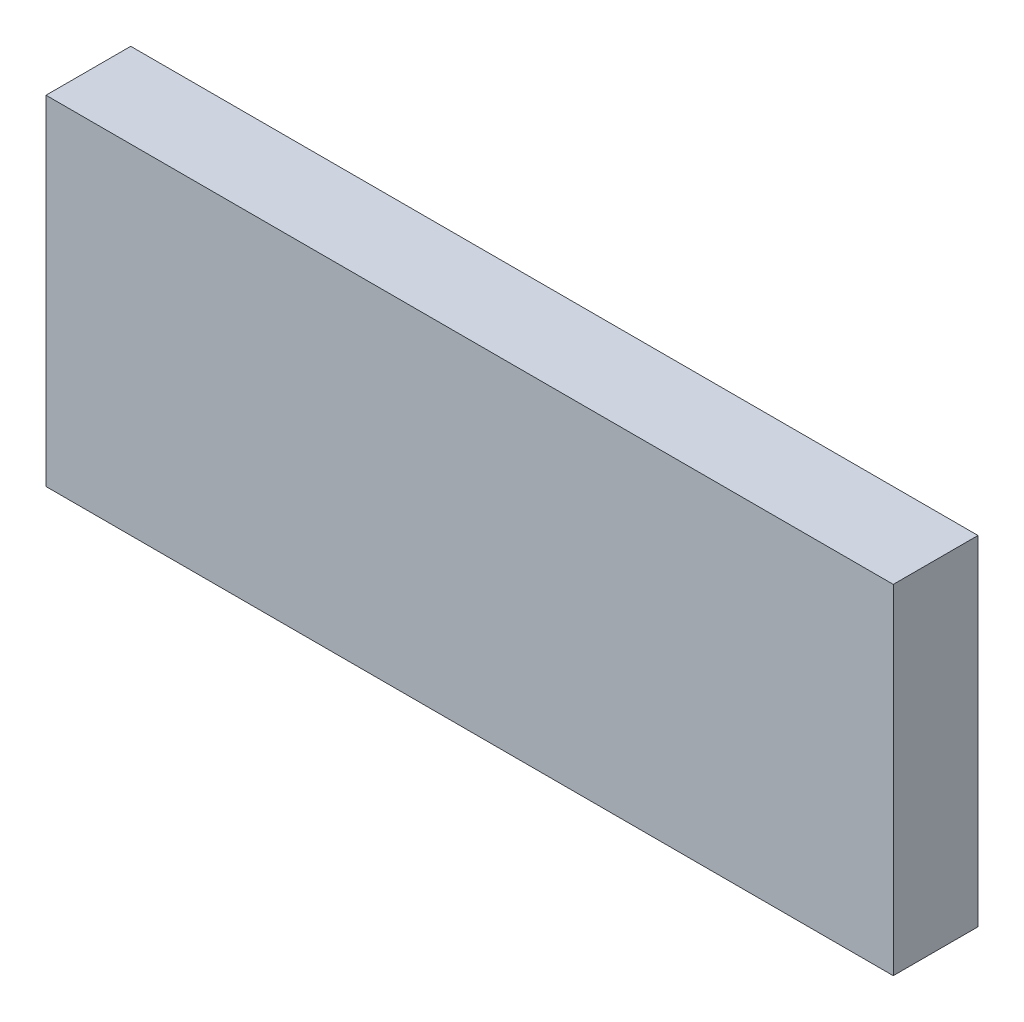
from build123d import *

# Parameters (mm, degrees)
SKETCH1_W           = 250
SKETCH1_H           = 100
BOSS_EXTRUDE1_DEPTH = 25


with BuildPart() as part:
    # Sketch1 → Boss-Extrude1 (new body)
    with BuildSketch(Plane.XY):
        with Locations((-125, 50)):
            Rectangle(SKETCH1_W, SKETCH1_H)
    extrude(amount=BOSS_EXTRUDE1_DEPTH)


solid = part.part
